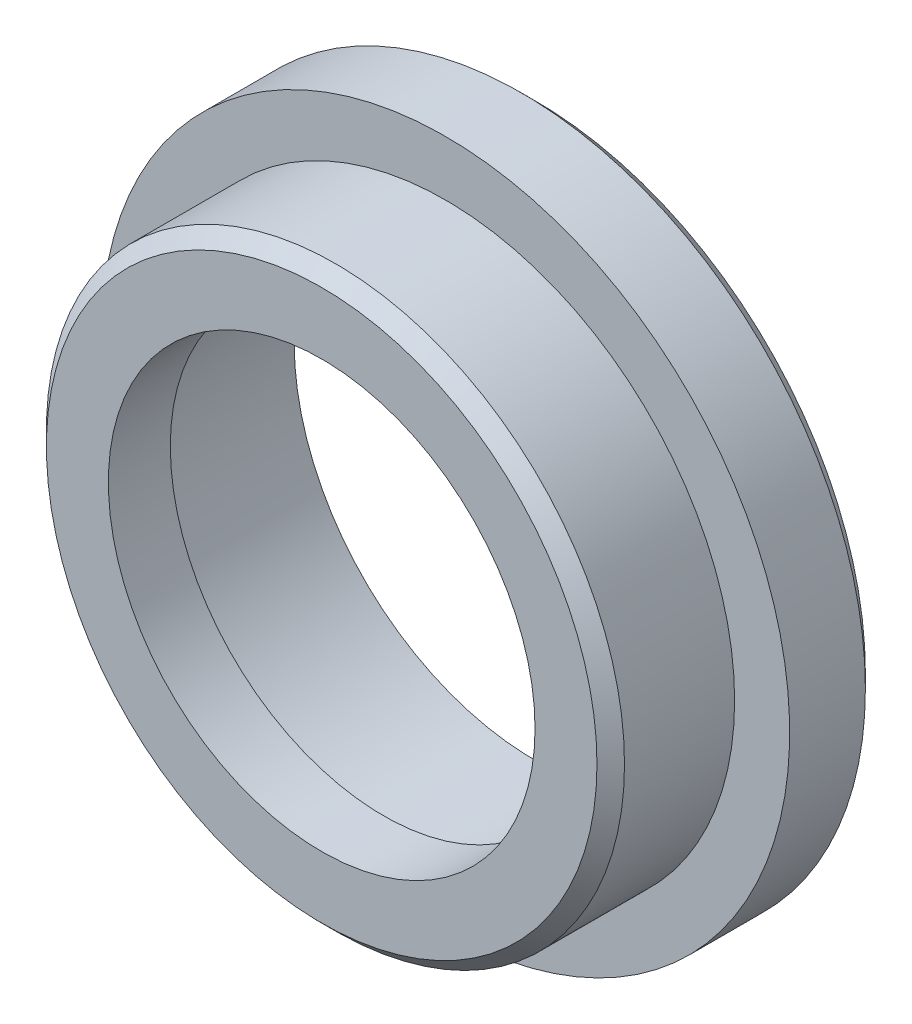
from build123d import *

# Parameters (mm, degrees)
SKETCH1_R           = 25
BOSS_EXTRUDE1_DEPTH = 6.5
SKETCH2_R           = 21
BOSS_EXTRUDE3_DEPTH = 9
SKETCH5_R           = 15.5
CUT_EXTRUDE2_DEPTH  = 43
SKETCH6_R           = 17.5
CUT_EXTRUDE3_DEPTH  = 11
SKETCH7_R           = 17.5
SKETCH7_R_2         = 16.5
CUT_EXTRUDE4_DEPTH  = 0.5
CHAMFER1_SIZE       = 1


with BuildPart() as part:
    # Sketch1 → Boss-Extrude1 (new body)
    with BuildSketch(Plane.XY):
        with Locations(Location((0, 0, 0), (0, 0, 180))):
            Circle(SKETCH1_R)
    extrude(amount=BOSS_EXTRUDE1_DEPTH)

    # Sketch2 → Boss-Extrude3 (add)
    with BuildSketch(Plane.XY.offset(6.5)):
        Circle(SKETCH2_R)
    extrude(amount=BOSS_EXTRUDE3_DEPTH)

    # Sketch5 → Cut-Extrude2 (cut)
    with BuildSketch(Plane.XY.offset(15.5)):
        Circle(SKETCH5_R)
    extrude(amount=-CUT_EXTRUDE2_DEPTH, mode=Mode.SUBTRACT)

    # Sketch6 → Cut-Extrude3 (cut)
    with BuildSketch(Plane(origin=(0, 0, 0), x_dir=(-1, 0, 0), z_dir=(0, 0, -1))):
        Circle(SKETCH6_R)
    extrude(amount=-CUT_EXTRUDE3_DEPTH, mode=Mode.SUBTRACT)

    # Sketch7 → Cut-Extrude4 (cut)
    with BuildSketch(Plane(origin=(0, 0, 11), x_dir=(-1, 0, 0), z_dir=(0, 0, -1))):
        Circle(SKETCH7_R)
        Circle(SKETCH7_R_2, mode=Mode.SUBTRACT)
    extrude(amount=-CUT_EXTRUDE4_DEPTH, mode=Mode.SUBTRACT)

    # Chamfer1
    chamfer1_edges = [part.edges().sort_by_distance(p)[0] for p in [
        (25, 0, 0),
        (-21, 0, 15.5),
    ]]
    chamfer(chamfer1_edges, length=CHAMFER1_SIZE)


solid = part.part
